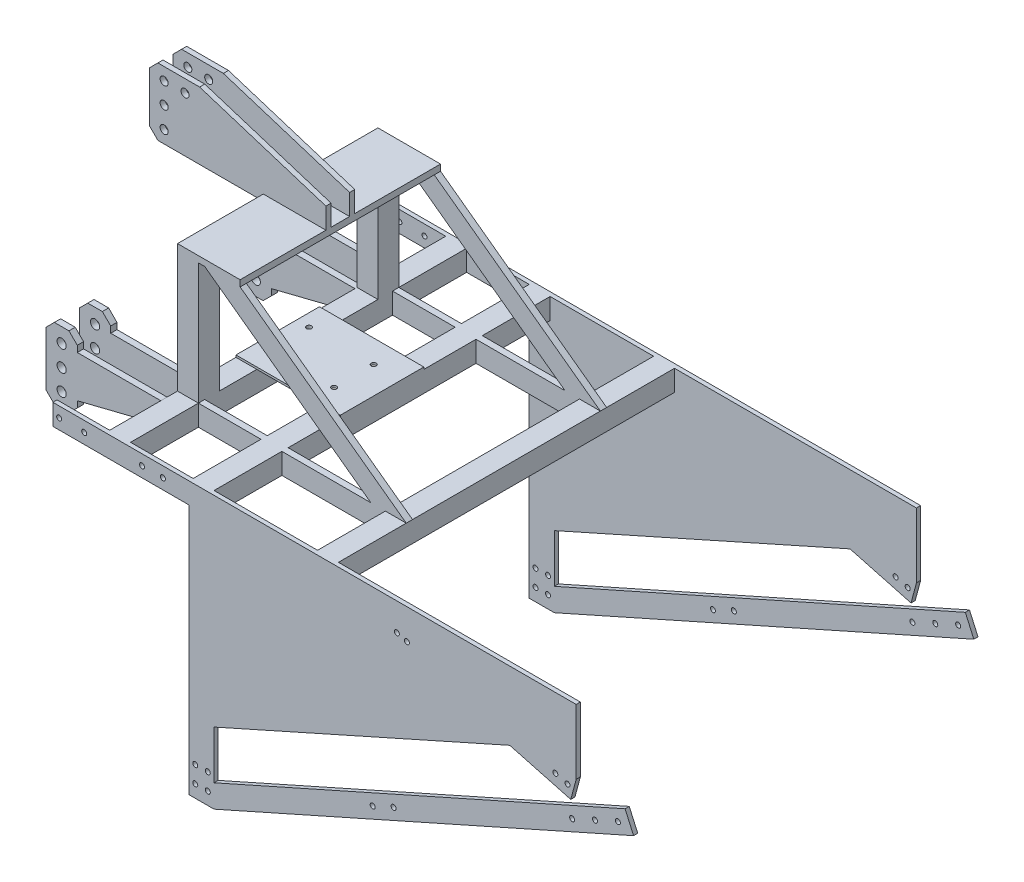
from build123d import *
from build123d.topology import SkipClean

# Parameters (mm, degrees)
SKETCH_1_W           = 50
SKETCH_1_H           = 50
SKETCH_1_W_2         = 40
SKETCH_1_H_2         = 40
EXTRUDE_1_DEPTH      = 402.5
SKETCH_2_R           = 6
EXTRUDE_2_DEPTH      = 10
SKETCH_3_W           = 50
SKETCH_3_H           = 50
SKETCH_3_W_2         = 40
SKETCH_3_H_2         = 40
EXTRUDE_3_DEPTH      = 805
EXTRUDE_START        = 10
SKETCH_4_R           = 6
EXTRUDE_4_DEPTH      = 10
SKETCH_5_R           = 11
EXTRUDE_5_DEPTH      = 47.5
SKETCH_7_R           = 11
EXTRUDE_6_DEPTH      = 47.5
SKETCH_10_W          = 350.5429373
SKETCH_10_H          = 65
CUT_EXTRUDE_6_DEPTH  = 1113.707453763
SKETCH_11_W          = 50
SKETCH_11_H          = 50
SKETCH_11_W_2        = 40
SKETCH_11_H_2        = 40
EXTRUDE_7_DEPTH      = 805
SKETCH_12_W          = 315.627196555
SKETCH_12_H          = 65
CUT_EXTRUDE_7_DEPTH  = 1113.707453763
SKETCH_13_W          = 447.894318558
SKETCH_13_H          = 50
EXTRUDE_8_DEPTH      = 7.5
SKETCH_14_W          = 447.894318558
SKETCH_14_H          = 50
EXTRUDE_9_DEPTH      = 7.5
SKETCH_15_R          = 9.65
EXTRUDE_10_DEPTH     = 34.5
SKETCH_16_W          = 600.562812098
SKETCH_16_H          = 44.5
CUT_EXTRUDE_8_DEPTH  = 200
SKETCH_19_W          = 480
SKETCH_19_H          = 15
EXTRUDE_11_DEPTH     = 200
EXTRUDE_12_DEPTH     = 15
EXTRUDE_13_DEPTH     = 15
SKETCH_23_W          = 50
SKETCH_23_H          = 50
SKETCH_23_W_2        = 40
SKETCH_23_H_2        = 40
EXTRUDE_14_DEPTH     = 291
CUT_EXTRUDE_9_DEPTH  = 1177.572512708
SKETCH_25_R          = 6
EXTRUDE_15_DEPTH     = 5
SKETCH_26_R          = 6
CUT_EXTRUDE_10_DEPTH = 1095.466937673
EXTRUDE_START_2      = -10
SKETCH_27_R          = 6
EXTRUDE_16_DEPTH     = 10
SKETCH_29_R          = 6
EXTRUDE_17_DEPTH     = 10
SKETCH_30_R          = 6
EXTRUDE_18_DEPTH     = 10
SKETCH_31_R          = 6
EXTRUDE_19_DEPTH     = 10
EXTRUDE_21_DEPTH     = 10
EXTRUDE_23_DEPTH     = 10
EXTRUDE_26_DEPTH     = 10
EXTRUDE_28_DEPTH     = 10
EXTRUDE_29_DEPTH     = 10
EXTRUDE_30_DEPTH     = 10


with BuildPart() as part:
    # 草图1 → 凸台-拉伸1 (new, symmetric)
    with BuildSketch(Plane.XY):
        with Locations((25, 25)):
            Rectangle(SKETCH_1_W, SKETCH_1_H)
        with Locations((25, 25)):
            Rectangle(SKETCH_1_W_2, SKETCH_1_H_2, mode=Mode.SUBTRACT)
    extrude(amount=EXTRUDE_1_DEPTH, both=True)

    # 草图2 → 凸台-拉伸2 (add)
    with BuildSketch(Plane.XY.offset(402.5)):
        Polygon((-237.894318558, -601), (767.005684849, -153.589692617), (746.668852695, -107.912419734), (-237.894318558, -546.268186075), (-237.894318558, 0), (43.417375121, 0), (616.614543518, -153.587718376), (629.555495773, -105.291427062), (50, 50), (-250, 50), (-297.894318558, 50), (-497.894318558, 50), (-577.894318558, 50), (-623.894318558, 50), (-623.894318558, 0), (-577.894318558, 0), (-497.894318558, 0), (-297.894318558, 0), (-297.894318558, -601), align=None)
        with Locations((-282.894318558, -531)):
            Circle(SKETCH_2_R, mode=Mode.SUBTRACT)
        with Locations((-252.894318558, -531)):
            Circle(SKETCH_2_R, mode=Mode.SUBTRACT)
        with Locations((-282.894318558, -571)):
            Circle(SKETCH_2_R, mode=Mode.SUBTRACT)
        with Locations((-252.894318558, -571)):
            Circle(SKETCH_2_R, mode=Mode.SUBTRACT)
        with Locations((142.105681442, -404.44719262)):
            Circle(SKETCH_2_R, mode=Mode.SUBTRACT)
        with Locations((-267.894318558, -248)):
            Circle(SKETCH_2_R, mode=Mode.SUBTRACT)
        with Locations((-267.894318558, -284)):
            Circle(SKETCH_2_R, mode=Mode.SUBTRACT)
        with Locations((192.105681442, -382.185758355)):
            Circle(SKETCH_2_R, mode=Mode.SUBTRACT)
        with Locations((729.430905043, -142.953155468)):
            Circle(SKETCH_2_R, mode=Mode.SUBTRACT)
        with Locations((674.618177584, -167.357354052)):
            Circle(SKETCH_2_R, mode=Mode.SUBTRACT)
        with Locations((619.805450126, -191.761552637)):
            Circle(SKETCH_2_R, mode=Mode.SUBTRACT)
        with Locations((608.596132252, -125.557287042)):
            Circle(SKETCH_2_R, mode=Mode.SUBTRACT)
        with Locations((579.618357463, -117.792715689)):
            Circle(SKETCH_2_R, mode=Mode.SUBTRACT)
        with Locations((-608.894318558, 25)):
            Circle(SKETCH_2_R, mode=Mode.SUBTRACT)
        with Locations((-548.894318558, 25)):
            Circle(SKETCH_2_R, mode=Mode.SUBTRACT)
        with Locations((-360.394318558, 25)):
            Circle(SKETCH_2_R, mode=Mode.SUBTRACT)
        with Locations((-410.394318558, 25)):
            Circle(SKETCH_2_R, mode=Mode.SUBTRACT)
        with Locations((200, -16.074283375)):
            Circle(SKETCH_2_R, mode=Mode.SUBTRACT)
        with Locations((224.148145657, -22.544759502)):
            Circle(SKETCH_2_R, mode=Mode.SUBTRACT)
    extrude(amount=EXTRUDE_2_DEPTH)

    # 草图3 → 凸台-拉伸3 (add)
    with BuildSketch(Plane(origin=(0, 0, 402.5), x_dir=(-1, 0, 0), z_dir=(0, 0, -1))):
        with Locations((272.894318558, 25)):
            Rectangle(SKETCH_3_W, SKETCH_3_H)
        with Locations((272.894318558, 25)):
            Rectangle(SKETCH_3_W_2, SKETCH_3_H_2, mode=Mode.SUBTRACT)
    extrude(amount=EXTRUDE_3_DEPTH)

    # 草图4 → 凸台-拉伸4 (add)
    with BuildSketch(Plane(origin=(0, 0, -402.5), x_dir=(-1, 0, 0), z_dir=(0, 0, -1)).offset(EXTRUDE_START)):
        Polygon((-612.809780816, -100.804426262), (-50, 50), (297.894318558, 50), (497.894318558, 50), (577.894318558, 50), (623.894318558, 50), (623.894318558, 0), (577.894318558, 0), (497.894318558, 0), (297.894318558, 0), (297.894318558, -601), (237.894318558, -601), (-767.005684849, -153.589692617), (-746.668852695, -107.912419734), (237.894318558, -546.268186075), (237.894318558, 0), (-43.417375121, 0), (-616.614543518, -153.587718376), (-629.555495773, -105.291427062), align=None)
        with Locations(Location((267.894318558, -248, 0), (0, 0, 180))):
            Circle(SKETCH_4_R, mode=Mode.SUBTRACT)
        with Locations(Location((267.894318558, -284, 0), (0, 0, 180))):
            Circle(SKETCH_4_R, mode=Mode.SUBTRACT)
        with Locations(Location((252.894318558, -531, 0), (0, 0, 180))):
            Circle(SKETCH_4_R, mode=Mode.SUBTRACT)
        with Locations(Location((282.894318558, -531, 0), (0, 0, 180))):
            Circle(SKETCH_4_R, mode=Mode.SUBTRACT)
        with Locations(Location((282.894318558, -571, 0), (0, 0, 180))):
            Circle(SKETCH_4_R, mode=Mode.SUBTRACT)
        with Locations(Location((252.894318558, -571, 0), (0, 0, 180))):
            Circle(SKETCH_4_R, mode=Mode.SUBTRACT)
        with Locations(Location((-192.105681442, -382.185758355, 0), (0, 0, 180))):
            Circle(SKETCH_4_R, mode=Mode.SUBTRACT)
        with Locations(Location((-142.105681442, -404.44719262, 0), (0, 0, 180))):
            Circle(SKETCH_4_R, mode=Mode.SUBTRACT)
        with Locations(Location((-608.596132252, -125.557287042, 0), (0, 0, 180))):
            Circle(SKETCH_4_R, mode=Mode.SUBTRACT)
        with Locations(Location((-579.618357463, -117.792715689, 0), (0, 0, 180))):
            Circle(SKETCH_4_R, mode=Mode.SUBTRACT)
        with Locations(Location((-674.618177584, -167.357354052, 0), (0, 0, 180))):
            Circle(SKETCH_4_R, mode=Mode.SUBTRACT)
        with Locations(Location((-729.430905043, -142.953155468, 0), (0, 0, 180))):
            Circle(SKETCH_4_R, mode=Mode.SUBTRACT)
        with Locations(Location((-619.805450126, -191.761552637, 0), (0, 0, 180))):
            Circle(SKETCH_4_R, mode=Mode.SUBTRACT)
        with Locations(Location((608.894318558, 25, 0), (0, 0, 180))):
            Circle(SKETCH_4_R, mode=Mode.SUBTRACT)
        with Locations(Location((548.894318558, 25, 0), (0, 0, 180))):
            Circle(SKETCH_4_R, mode=Mode.SUBTRACT)
    extrude(amount=-EXTRUDE_4_DEPTH)



with BuildPart() as body_2:
    # 草图5 → 凸台-拉伸5 (new, symmetric)
    with BuildSketch(Plane.XY.offset(232.5)):
        Polygon((-497.894318558, 50), (-497.894318558, 0), (-697.894318558, -50), (-697.894318558, -65), (-717.894318558, -85), (-752.894318558, -85), (-772.894318558, -65), (-772.894318558, 65), (-752.894318558, 85), (-717.894318558, 85), (-697.894318558, 65), (-697.894318558, 50), align=None)
        with Locations((-735.394318558, 50)):
            Circle(SKETCH_5_R, mode=Mode.SUBTRACT)
        with Locations((-735.394318558, 0)):
            Circle(SKETCH_5_R, mode=Mode.SUBTRACT)
        with Locations((-735.394318558, -50)):
            Circle(SKETCH_5_R, mode=Mode.SUBTRACT)
    extrude(amount=EXTRUDE_5_DEPTH, both=True)

    # 草图12 → 切除-拉伸7 (cut, through all)
    with BuildSketch(Plane(origin=(0, 85, 0), x_dir=(1, 0, 0), z_dir=(0, 1, 0))):
        with Locations((-655.707916836, -232.5)):
            Rectangle(SKETCH_12_W, SKETCH_12_H)
    extrude(amount=-CUT_EXTRUDE_7_DEPTH, mode=Mode.SUBTRACT)


with BuildPart() as body_3:
    # 草图7 → 凸台-拉伸6 (new, symmetric)
    with BuildSketch(Plane.XY.offset(-232.5)):
        Polygon((-772.894318558, 65), (-772.894318558, -65), (-752.894318558, -85), (-717.894318558, -85), (-697.894318558, -65), (-697.894318558, -50), (-497.894318558, 0), (-497.894318558, 50), (-697.894318558, 50), (-697.894318558, 65), (-717.894318558, 85), (-752.894318558, 85), align=None)
        with Locations((-735.394318558, 50)):
            Circle(SKETCH_7_R, mode=Mode.SUBTRACT)
        with Locations((-735.394318558, 0)):
            Circle(SKETCH_7_R, mode=Mode.SUBTRACT)
        with Locations((-735.394318558, -50)):
            Circle(SKETCH_7_R, mode=Mode.SUBTRACT)
    extrude(amount=EXTRUDE_6_DEPTH, both=True)

    # 草图10 → 切除-拉伸6 (cut, through all)
    with BuildSketch(Plane(origin=(0, 85, 0), x_dir=(1, 0, 0), z_dir=(0, 1, 0))):
        with Locations((-629.704561359, 232.5)):
            Rectangle(SKETCH_10_W, SKETCH_10_H)
    extrude(amount=-CUT_EXTRUDE_6_DEPTH, mode=Mode.SUBTRACT)


with BuildPart() as cut_extrude_6_piece_1:
    # of the separate pieces the step leaves, piece 1, a body of its own (cut_extrude_6_pieces)
    add(body_3.part.solids().sort_by_distance((-772.894318558, 65, -265))[0])


with BuildPart() as cut_extrude_6_piece_2:
    # of the separate pieces the step leaves, piece 2, a body of its own (cut_extrude_6_pieces)
    add(body_3.part.solids().sort_by_distance((-772.894318558, 65, -185))[0])


with BuildPart() as part_1:
    add(part.part)

    add(cut_extrude_6_piece_1.part)  # 凸台-拉伸7 merges 切除-拉伸6 piece 1

    add(cut_extrude_6_piece_2.part)  # 凸台-拉伸7 merges 切除-拉伸6 piece 2
    # 草图11 → 凸台-拉伸7 (add)
    with BuildSketch(Plane.XY.offset(-402.5)):
        with Locations((-472.894318558, 25)):
            Rectangle(SKETCH_11_W, SKETCH_11_H)
        with Locations((-472.894318558, 25.387152579)):
            Rectangle(SKETCH_11_W_2, SKETCH_11_H_2, mode=Mode.SUBTRACT)
    extrude(amount=EXTRUDE_7_DEPTH)

    # 草图13 → 凸台-拉伸8 (add, symmetric)
    with BuildSketch(Plane.XY.offset(232.5)):
        with Locations((-223.947159279, 25)):
            Rectangle(SKETCH_13_W, SKETCH_13_H)
    extrude(amount=EXTRUDE_8_DEPTH, both=True)

    # 草图14 → 凸台-拉伸9 (add, symmetric)
    with BuildSketch(Plane.XY.offset(-232.5)):
        with Locations((-223.947159279, 25)):
            Rectangle(SKETCH_14_W, SKETCH_14_H)
    extrude(amount=EXTRUDE_9_DEPTH, both=True)



with BuildPart() as cut_extrude_7_piece_1:
    # of the separate pieces the step leaves, piece 1, a body of its own (cut_extrude_7_pieces)
    add(body_2.part.solids().sort_by_distance((-497.894318558, 50, 185))[0])


with BuildPart() as cut_extrude_7_piece_2:
    # of the separate pieces the step leaves, piece 2, a body of its own (cut_extrude_7_pieces)
    add(body_2.part.solids().sort_by_distance((-497.894318558, 50, 265))[0])


with BuildPart() as body_4:
    # 草图15 → 凸台-拉伸10 (new, symmetric)
    with BuildSketch(Plane.XY):
        Polygon((-670.394318558, 341), (-297.894318558, 341), (-297.894318558, 404.924528302), (-645.394318558, 501.7), (-750.394318558, 501.7), (-770.394318558, 481.7), (-770.394318558, 371), (-770.394318558, 361), (-750.394318558, 341), align=None)
        with Locations((-735.394318558, 471.7)):
            Circle(SKETCH_15_R, mode=Mode.SUBTRACT)
        with Locations((-735.394318558, 371)):
            Circle(SKETCH_15_R, mode=Mode.SUBTRACT)
        with Locations((-735.394318558, 421.7)):
            Circle(SKETCH_15_R, mode=Mode.SUBTRACT)
        with Locations((-685.394318558, 471.7)):
            Circle(SKETCH_15_R, mode=Mode.SUBTRACT)
    extrude(amount=EXTRUDE_10_DEPTH, both=True)

    # 草图16 → 切除-拉伸8 (cut)
    with BuildSketch(Plane(origin=(0, 501.7, 0), x_dir=(1, 0, 0), z_dir=(0, 1, 0))):
        with Locations((-521.376665995, 0)):
            Rectangle(SKETCH_16_W, SKETCH_16_H)
    extrude(amount=-CUT_EXTRUDE_8_DEPTH, mode=Mode.SUBTRACT)


with BuildPart() as cut_extrude_8_piece_1:
    # of the separate pieces the step leaves, piece 1, a body of its own (cut_extrude_8_pieces)
    add(body_4.part.solids().sort_by_distance((-750.394318558, 341, 22.25))[0])



with BuildPart() as cut_extrude_8_piece_2:
    # of the separate pieces the step leaves, piece 2, a body of its own (cut_extrude_8_pieces)
    add(body_4.part.solids().sort_by_distance((-750.394318558, 341, -34.5))[0])


with BuildPart() as cut_extrude_8_piece_1_1:
    add(cut_extrude_8_piece_1.part)

    add(cut_extrude_8_piece_2.part)  # 凸台-拉伸11 merges 切除-拉伸8 piece 2
    # 草图19 → 凸台-拉伸11 (add)
    with BuildSketch(Plane.ZY.offset(497.894318558)):
        with Locations((0, 348.5)):
            Rectangle(SKETCH_19_W, SKETCH_19_H)
    extrude(amount=-EXTRUDE_11_DEPTH)

    # 草图20 → 凸台-拉伸12 (add)
    with BuildSketch(Plane.XY.offset(240)):
        Polygon((-347.894318558, 341), (50, 50), (-34.699519451, 50), (-432.593838009, 341), align=None)
    extrude(amount=-EXTRUDE_12_DEPTH)

    # 草图21 → 凸台-拉伸13 (add)
    with BuildSketch(Plane.XY.offset(-225)):
        Polygon((50, 50), (-347.894318558, 341), (-432.593838009, 341), (-34.699519451, 50), align=None)
    extrude(amount=-EXTRUDE_13_DEPTH)


with BuildPart() as part_2:
    add(part_1.part)

    add(cut_extrude_7_piece_1.part)  # 凸台-拉伸14 merges 切除-拉伸7 piece 1

    add(cut_extrude_8_piece_1_1.part)  # 凸台-拉伸14 merges 切除-拉伸8 piece 1
    # 草图23 → 凸台-拉伸14 (add)
    # profile 1 of 2: a face of its own
    with BuildSketch(Plane(origin=(0, 50, 0), x_dir=(1, 0, 0), z_dir=(0, 1, 0))):
        with Locations((-472.894318558, -215)):
            Rectangle(SKETCH_23_W, SKETCH_23_H)
        with Locations((-472.894318558, -215)):
            Rectangle(SKETCH_23_W_2, SKETCH_23_H_2, mode=Mode.SUBTRACT)
    # profile 2 of 2: a face of its own
    with BuildSketch(Plane(origin=(0, 50, 0), x_dir=(1, 0, 0), z_dir=(0, 1, 0))):
        with Locations((-472.894318558, 215)):
            Rectangle(SKETCH_23_W, SKETCH_23_H)
        with Locations((-472.894318558, 215)):
            Rectangle(SKETCH_23_W_2, SKETCH_23_H_2, mode=Mode.SUBTRACT)
    extrude(amount=EXTRUDE_14_DEPTH)

    # 草图24 → 切除-拉伸9 (cut, through all)
    with BuildSketch(Plane.XY.offset(240)):
        Polygon((-347.894318558, 341), (-347.894318558, 356), (-347.894318558, 406), (-650.394318558, 501.7), (-650.394318558, 527.436827737), (-259.970201777, 527.436827737), (-259.970201777, 501.7), (-259.970201777, 341), align=None)
    extrude(amount=-CUT_EXTRUDE_9_DEPTH, mode=Mode.SUBTRACT)

    # 草图25 → 凸台-拉伸15 (add)
    with BuildSketch(Plane(origin=(0, 50, 0), x_dir=(1, 0, 0), z_dir=(0, 1, 0))):
        Polygon((-447.894318558, 100), (-247.894318558, 100), (-247.894318558, -100), (-454.686495764, -100), (-497.894318558, -100), (-497.894318558, 100), align=None)
        with Locations(Location((-467.894318558, 45, 0), (0, 0, 180))):
            Circle(SKETCH_25_R, mode=Mode.SUBTRACT)
        with Locations(Location((-312.894318558, 45, 0), (0, 0, 180))):
            Circle(SKETCH_25_R, mode=Mode.SUBTRACT)
        with Locations(Location((-312.894318558, -50, 0), (0, 0, 180))):
            Circle(SKETCH_25_R, mode=Mode.SUBTRACT)
        with Locations(Location((-467.894318558, -50, 0), (0, 0, 180))):
            Circle(SKETCH_25_R, mode=Mode.SUBTRACT)
    extrude(amount=EXTRUDE_15_DEPTH)

    # 草图26 → 切除-拉伸10 (cut, through all)
    with SkipClean():  # the faces are left unmerged after this step: merging them gives an invalid solid
        with BuildSketch(Plane(origin=(0, 55, 0), x_dir=(1, 0, 0), z_dir=(0, 1, 0))):
            with Locations((-467.894318558, -50)):
                Circle(SKETCH_26_R)
            with Locations((-467.894318558, 45)):
                Circle(SKETCH_26_R)
        extrude(amount=-CUT_EXTRUDE_10_DEPTH, mode=Mode.SUBTRACT)

    # 草图27 → 凸台-拉伸16 (add)
    with SkipClean():  # the faces are left unmerged after this step: merging them gives an invalid solid
        with BuildSketch(Plane.XY.offset(412.5).offset(EXTRUDE_START_2)):
            with Locations(Location((-267.894318558, -248, 0), (0, 0, 180))):
                Circle(SKETCH_27_R)
        extrude(amount=EXTRUDE_16_DEPTH)

    # 草图29 → 凸台-拉伸17 (add)
    with SkipClean():  # the faces are left unmerged after this step: merging them gives an invalid solid
        with BuildSketch(Plane.XY.offset(412.5).offset(EXTRUDE_START_2)):
            with Locations(Location((-267.894318558, -284, 0), (0, 0, 180))):
                Circle(SKETCH_29_R)
        extrude(amount=EXTRUDE_17_DEPTH)

    # 草图30 → 凸台-拉伸18 (add)
    with SkipClean():  # the faces are left unmerged after this step: merging them gives an invalid solid
        with BuildSketch(Plane(origin=(0, 0, -412.5), x_dir=(-1, 0, 0), z_dir=(0, 0, -1))):
            with Locations((267.894318558, -248)):
                Circle(SKETCH_30_R)
        extrude(amount=-EXTRUDE_18_DEPTH)

    # 草图31 → 凸台-拉伸19 (add)
    with SkipClean():  # the faces are left unmerged after this step: merging them gives an invalid solid
        with BuildSketch(Plane(origin=(0, 0, -412.5), x_dir=(-1, 0, 0), z_dir=(0, 0, -1))):
            with Locations((267.894318558, -284)):
                Circle(SKETCH_31_R)
        extrude(amount=-EXTRUDE_19_DEPTH)

    # 草图32 → 凸台-拉伸21 (add)
    with SkipClean():  # the faces are left unmerged after this step: merging them gives an invalid solid
        with BuildSketch(Plane.XY.offset(412.5)):
            Polygon((-237.894318558, 0), (-237.894318558, -400.6751023), (429.614248803, -103.481140422), (43.417375121, 0), align=None)
        extrude(amount=-EXTRUDE_21_DEPTH)

    # 草图33 → 凸台-拉伸23 (add)
    with SkipClean():  # the faces are left unmerged after this step: merging them gives an invalid solid
        with BuildSketch(Plane(origin=(0, 0, -412.5), x_dir=(-1, 0, 0), z_dir=(0, 0, -1))):
            Polygon((237.894318558, 0), (237.894318558, -400.6751023), (-429.614248803, -103.481140422), (-50, 0), align=None)
        extrude(amount=-EXTRUDE_23_DEPTH)

    # 草图34 → 凸台-拉伸26 (add)
    with SkipClean():  # the faces are left unmerged after this step: merging them gives an invalid solid
        with BuildSketch(Plane.XY.offset(412.5)):
            Polygon((50, 50), (629.555495773, -105.291427062), (629.555495773, 50), align=None)
        extrude(amount=-EXTRUDE_26_DEPTH)

    # 草图35 → 凸台-拉伸28 (add)
    with SkipClean():  # the faces are left unmerged after this step: merging them gives an invalid solid
        with BuildSketch(Plane(origin=(0, 0, -412.5), x_dir=(-1, 0, 0), z_dir=(0, 0, -1))):
            Polygon((-629.555495773, -105.291427062), (-629.555495773, 50), (-50, 50), align=None)
        extrude(amount=-EXTRUDE_28_DEPTH)

    # 草图36 → 凸台-拉伸29 (add)
    with SkipClean():  # the faces are left unmerged after this step: merging them gives an invalid solid
        with BuildSketch(Plane.XY.offset(412.5)):
            Polygon((-237.894318558, -400.6751023), (-237.894318558, -430.6751023), (470.46066832, -114.425905546), (429.614248803, -103.481140422), align=None)
        extrude(amount=-EXTRUDE_29_DEPTH)

    # 草图37 → 凸台-拉伸30 (add)
    with SkipClean():  # the faces are left unmerged after this step: merging them gives an invalid solid
        with BuildSketch(Plane(origin=(0, 0, -412.5), x_dir=(-1, 0, 0), z_dir=(0, 0, -1))):
            Polygon((237.894318558, -400.6751023), (237.894318558, -430.6751023), (-470.46066832, -114.425905546), (-429.614248803, -103.481140422), align=None)
        extrude(amount=-EXTRUDE_30_DEPTH)


solid = Compound([cut_extrude_7_piece_2.part, part_2.part])
